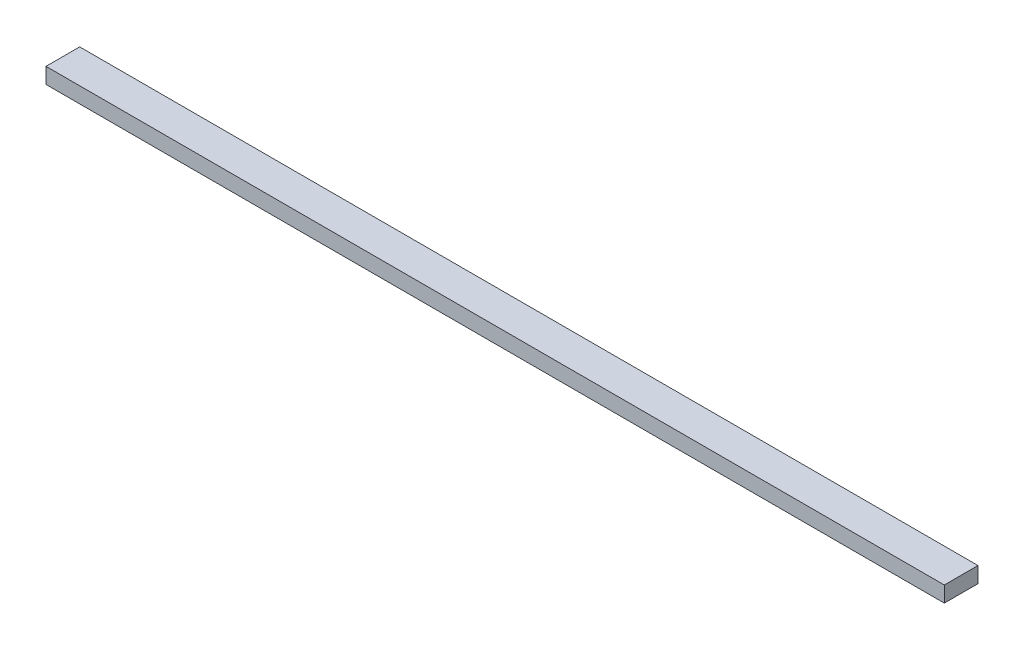
from build123d import *

# Parameters (mm, degrees)
SKETCH_1_W      = 800
SKETCH_1_H      = 14
EXTRUDE_1_DEPTH = 30


with BuildPart() as part:
    # 草图1 → 凸台-拉伸1 (new body)
    with BuildSketch(Plane.XY):
        Rectangle(SKETCH_1_W, SKETCH_1_H)
    extrude(amount=EXTRUDE_1_DEPTH)


solid = part.part
